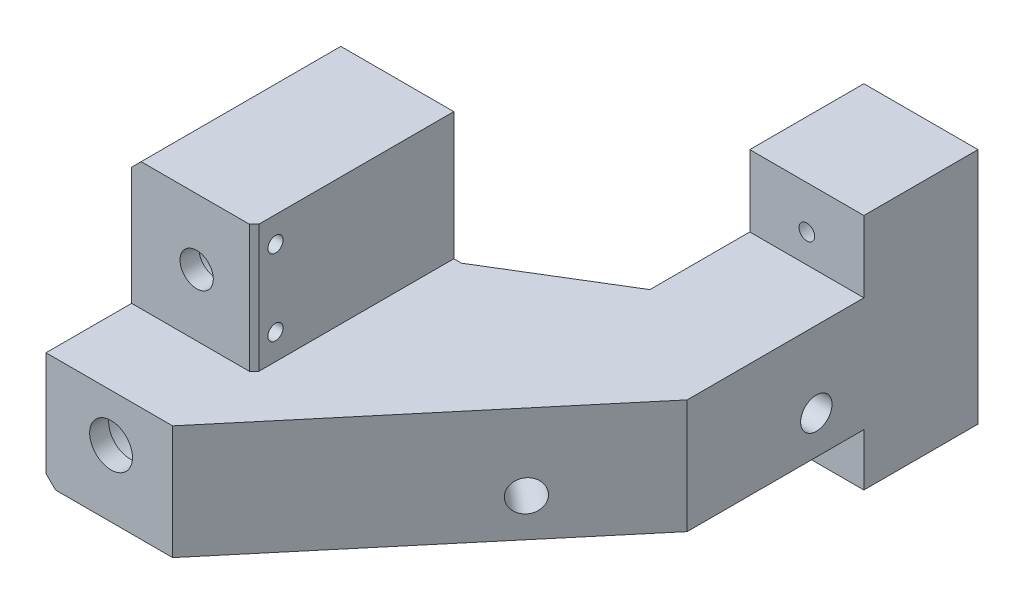
from build123d import *

# Parameters (mm, degrees)
BOSS_EXTRUDE1_DEPTH          = 26
SKETCH2_W                    = 36.317151105
SKETCH2_H                    = 12
CUT_EXTRUDE1_DEPTH           = 77
SKETCH3_R                    = 4
SKETCH3_R_2                  = 3.5
CUT_EXTRUDE2_DEPTH           = 50
SKETCH4_R                    = 4
SKETCH4_R_2                  = 2.25
BOSS_EXTRUDE2_DEPTH          = 2
SKETCH5_W                    = 9
SKETCH5_H                    = 21.000830638
CUT_EXTRUDE3_DEPTH           = 15
SKETCH6_R                    = 3.5
SKETCH6_R_2                  = 1.75
BOSS_EXTRUDE3_DEPTH          = 2
SKETCH10_W                   = 14.150971585
SKETCH10_H                   = 19.243046766
CUT_EXTRUDE4_DEPTH           = 60
SKETCH12_W                   = 13
SKETCH12_H                   = 24
BOSS_EXTRUDE6_DEPTH          = 12
SKETCH13_W                   = 1
SKETCH13_H                   = 22.5
CUT_EXTRUDE6_DEPTH           = 75.966659256
CUT_EXTRUDE7_DEPTH           = 35
CUT_EXTRUDE10_DEPTH          = 2
SKETCH19_W                   = 12
SKETCH19_H                   = 5.5
BOSS_EXTRUDE7_DEPTH          = 12
SKETCH20_W                   = 12
SKETCH20_H                   = 4.5
CUT_EXTRUDE11_DEPTH          = 14.6
SKETCH7_W                    = 13.682848895
SKETCH7_H                    = 21
CUT_EXTRUDE9_DEPTH           = 0.6
SKETCH21_W                   = 21
SKETCH21_H                   = 13.4
CUT_EXTRUDE12_DEPTH          = 0.8
M4_TAPPED_HOLE1_D            = 3.3
M4_TAPPED_HOLE1_DEPTH        = 11.5
M4_TAPPED_HOLE1_TIP          = 0.991420021
M2_TAPPED_HOLE1_D            = 1.6
M2_TAPPED_HOLE1_DEPTH        = 6
M2_TAPPED_HOLE1_TIP          = 0.480688495
F_3_0_3_DIAMETER_HOLE1_D     = 3
F_3_0_3_DIAMETER_HOLE1_DEPTH = 8
F_3_0_3_DIAMETER_HOLE1_TIP   = 0.901290929
CHAMFER1_SIZE                = 0.5
M4_TAPPED_HOLE2_D            = 3.3
M4_TAPPED_HOLE2_DEPTH        = 10
M4_TAPPED_HOLE2_TIP          = 0.991420021
M4_TAPPED_HOLE3_D            = 3.3
M4_TAPPED_HOLE3_DEPTH        = 11.5
M4_TAPPED_HOLE3_TIP          = 0.991420021
CHAMFER2_SIZE                = 1


with BuildPart() as part:
    # Sketch1 → Boss-Extrude1 (new body)
    with BuildSketch(Plane(origin=(0, 0, 0), x_dir=(1, 0, 0), z_dir=(0, 1, 0))):
        Polygon((24, 0), (50, 40), (50, 60), (25, 60), (25, 47.4110017), (13.682848895, 30), (0, 30), (0, 0), align=None)
    extrude(amount=BOSS_EXTRUDE1_DEPTH)

    # Sketch2 → Cut-Extrude1 (cut)
    with BuildSketch(Plane(origin=(0, 0, -60), x_dir=(-1, 0, 0), z_dir=(0, 0, -1))):
        with Locations((-31.841424447, 20)):
            Rectangle(SKETCH2_W, SKETCH2_H)
    extrude(amount=-CUT_EXTRUDE1_DEPTH, mode=Mode.SUBTRACT)

    # Sketch3 → Cut-Extrude2 (cut)
    with BuildSketch(Plane.XY):
        with Locations((6.841424448, 7)):
            Circle(SKETCH3_R)
        with Locations((6.841424448, 18.5)):
            Circle(SKETCH3_R_2)
    extrude(amount=-CUT_EXTRUDE2_DEPTH, mode=Mode.SUBTRACT)

    # Sketch4 → Boss-Extrude2 (add)
    with BuildSketch(Plane.XY):
        with Locations((6.841424448, 7)):
            Circle(SKETCH4_R)
        with Locations((6.841424448, 7)):
            Circle(SKETCH4_R_2, mode=Mode.SUBTRACT)
    extrude(amount=-BOSS_EXTRUDE2_DEPTH)

    # Sketch5 → Cut-Extrude3 (cut)
    with BuildSketch(Plane.ZY):
        with Locations((-4.5, 22.500415319)):
            Rectangle(SKETCH5_W, SKETCH5_H)
    extrude(amount=-CUT_EXTRUDE3_DEPTH, mode=Mode.SUBTRACT)

    # Sketch6 → Boss-Extrude3 (add)
    with BuildSketch(Plane.XY.offset(-9)):
        with Locations((6.841424448, 18.5)):
            Circle(SKETCH6_R)
        with Locations((6.841424448, 18.5)):
            Circle(SKETCH6_R_2, mode=Mode.SUBTRACT)
    extrude(amount=-BOSS_EXTRUDE3_DEPTH)

    # Sketch10 → Cut-Extrude4 (cut)
    with BuildSketch(Plane(origin=(0, 0, -60), x_dir=(-1, 0, 0), z_dir=(0, 0, -1))):
        with Locations((-45.075485793, 9.621523383)):
            Rectangle(SKETCH10_W, SKETCH10_H)
    extrude(amount=-CUT_EXTRUDE4_DEPTH, mode=Mode.SUBTRACT)

    # Sketch12 → Boss-Extrude6 (add)
    with BuildSketch(Plane(origin=(0, 0, -60), x_dir=(-1, 0, 0), z_dir=(0, 0, -1))):
        with Locations((-31.5, 12)):
            Rectangle(SKETCH12_W, SKETCH12_H)
    extrude(amount=-BOSS_EXTRUDE6_DEPTH)

    # Sketch13 → Cut-Extrude6 (cut, through all)
    with BuildSketch(Plane(origin=(0, 24, 0), x_dir=(1, 0, 0), z_dir=(0, 1, 0))):
        with Locations((25.5, 48.75)):
            Rectangle(SKETCH13_W, SKETCH13_H)
    extrude(amount=-CUT_EXTRUDE6_DEPTH, mode=Mode.SUBTRACT)

    # Sketch15 → Cut-Extrude7 (cut)
    with BuildSketch(Plane(origin=(0, 14, 0), x_dir=(1, 0, 0), z_dir=(0, 1, 0))):
        Polygon((13.682848895, 30), (26, 37.5), (26, 50.957252655), (13.682848895, 50.957252655), align=None)
        Polygon((13.312598457, 0), (38, 0), (38, 29.42129948), align=None)
    extrude(amount=-CUT_EXTRUDE7_DEPTH, mode=Mode.SUBTRACT)

    # Sketch18 → Cut-Extrude10 (cut)
    with BuildSketch(Plane(origin=(0, 14, 0), x_dir=(1, 0, 0), z_dir=(0, 1, 0))):
        Polygon((26, 48), (38, 48), (38, 29.42129948), (13.682848895, 0.44124729), (13.682848895, 30), (26, 37.5), align=None)
    extrude(amount=-CUT_EXTRUDE10_DEPTH, mode=Mode.SUBTRACT)

    # Sketch19 → Boss-Extrude7 (add)
    with BuildSketch(Plane(origin=(0, 0, -60), x_dir=(-1, 0, 0), z_dir=(0, 0, -1))):
        with Locations((-32, -2.75)):
            Rectangle(SKETCH19_W, SKETCH19_H)
    extrude(amount=-BOSS_EXTRUDE7_DEPTH)

    # Sketch20 → Cut-Extrude11 (cut)
    with BuildSketch(Plane(origin=(0, 0, -60), x_dir=(-1, 0, 0), z_dir=(0, 0, -1))):
        with Locations((-32, 21.75)):
            Rectangle(SKETCH20_W, SKETCH20_H)
    extrude(amount=-CUT_EXTRUDE11_DEPTH, mode=Mode.SUBTRACT)

    # Sketch7 → Cut-Extrude9 (cut)
    with BuildSketch(Plane(origin=(0, 26, 0), x_dir=(1, 0, 0), z_dir=(0, 1, 0))):
        with Locations((6.841424448, 19.5)):
            Rectangle(SKETCH7_W, SKETCH7_H)
    extrude(amount=-CUT_EXTRUDE9_DEPTH, mode=Mode.SUBTRACT)

    # Sketch21 → Cut-Extrude12 (cut)
    with BuildSketch(Plane(origin=(13.682848895, 0, 0), x_dir=(0, 0, -1), z_dir=(1, 0, 0))):
        with Locations((19.5, 18.7)):
            Rectangle(SKETCH21_W, SKETCH21_H)
    extrude(amount=-CUT_EXTRUDE12_DEPTH, mode=Mode.SUBTRACT)

    # M4 Tapped Hole1
    with Locations(Plane(origin=(0, 0, -60), x_dir=(-1, 0, 0), z_dir=(0, 0, -1))):
        with Locations((-32, 15), (-32, -1)):
            Hole(M4_TAPPED_HOLE1_D / 2, depth=M4_TAPPED_HOLE1_DEPTH)
            with Locations((0, 0, -(M4_TAPPED_HOLE1_DEPTH + M4_TAPPED_HOLE1_TIP / 2))):  # 118° drill point
                Cone(0, M4_TAPPED_HOLE1_D / 2, M4_TAPPED_HOLE1_TIP, mode=Mode.SUBTRACT)

    # M2 Tapped Hole1
    with Locations(Plane(origin=(12.882848895, 0, 0), x_dir=(0, 0, -1), z_dir=(1, 0, 0))):
        with Locations((11.25, 14.7), (11.25, 22.7)):
            Hole(M2_TAPPED_HOLE1_D / 2, depth=M2_TAPPED_HOLE1_DEPTH)
            with Locations((0, 0, -(M2_TAPPED_HOLE1_DEPTH + M2_TAPPED_HOLE1_TIP / 2))):  # 118° drill point
                Cone(0, M2_TAPPED_HOLE1_D / 2, M2_TAPPED_HOLE1_TIP, mode=Mode.SUBTRACT)

    # Ø3.0 (3) Diameter Hole1
    with Locations(Plane(origin=(0, 0, -60), x_dir=(-1, 0, 0), z_dir=(0, 0, -1))):
        with Locations((-32, 10), (-32, 4)):
            Hole(F_3_0_3_DIAMETER_HOLE1_D / 2, depth=F_3_0_3_DIAMETER_HOLE1_DEPTH)
            with Locations((0, 0, -(F_3_0_3_DIAMETER_HOLE1_DEPTH + F_3_0_3_DIAMETER_HOLE1_TIP / 2))):  # 118° drill point
                Cone(0, F_3_0_3_DIAMETER_HOLE1_D / 2, F_3_0_3_DIAMETER_HOLE1_TIP, mode=Mode.SUBTRACT)

    # Chamfer1
    chamfer1_edges = [part.edges().sort_by_distance(p)[0] for p in [
        (12.882848895, 18.7, -9),
    ]]
    chamfer(chamfer1_edges, length=CHAMFER1_SIZE)

    # M4 Tapped Hole2
    with Locations(Plane(origin=(38, 0, 0), x_dir=(0, 0, -1), z_dir=(1, 0, 0))):
        with Locations((43, 4)):
            Hole(M4_TAPPED_HOLE2_D / 2, depth=M4_TAPPED_HOLE2_DEPTH)
            with Locations((0, 0, -(M4_TAPPED_HOLE2_DEPTH + M4_TAPPED_HOLE2_TIP / 2))):  # 118° drill point
                Cone(0, M4_TAPPED_HOLE2_D / 2, M4_TAPPED_HOLE2_TIP, mode=Mode.SUBTRACT)

    # M4 Tapped Hole3
    with Locations(Plane(origin=(7.81215346, 0, 6.555175087), x_dir=(0.6427876096865373, 0, -0.7660444431189798), z_dir=(0.7660444431189798, 0, 0.6427876096865373))):
        with Locations((34.963952144, 4)):
            Hole(M4_TAPPED_HOLE3_D / 2, depth=M4_TAPPED_HOLE3_DEPTH)
            with Locations((0, 0, -(M4_TAPPED_HOLE3_DEPTH + M4_TAPPED_HOLE3_TIP / 2))):  # 118° drill point
                Cone(0, M4_TAPPED_HOLE3_D / 2, M4_TAPPED_HOLE3_TIP, mode=Mode.SUBTRACT)

    # Chamfer2
    chamfer2_edges = [part.edges().sort_by_distance(p)[0] for p in [
        (0, 0, -15),
        (0, 25.4, -19.5),
    ]]
    chamfer(chamfer2_edges, length=CHAMFER2_SIZE)


solid = part.part
